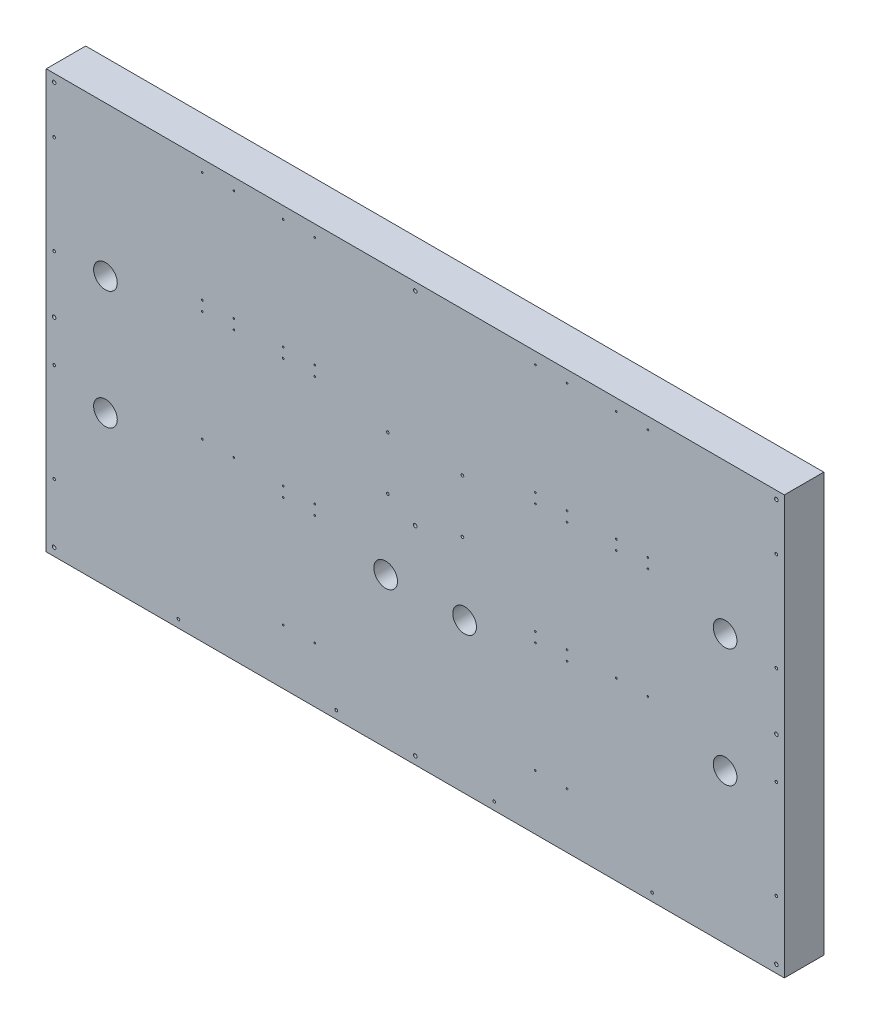
SolidWorks part; units mm, degrees
material "陶瓷"
ref_plane "前视基准面" through (0, 0, 0) normal (0, 0, 1) x (1, 0, 0)
ref_plane "上视基准面" through (0, 0, 0) normal (0, 1, 0) x (1, 0, 0)
ref_plane "右视基准面" through (0, 0, 0) normal (1, 0, 0) x (0, 0, -1)
sketch "草图1" plane through (0, 0, 0) normal (0, 0, 1) x (1, 0, 0)
  line L1 (-935, -530) -> (935, -530)
  line L2 (-935, -530) -> (-935, 530)
  line L3 (-935, 530) -> (935, 530)
  line L4 (935, -530) -> (935, 530)
  line L5 (-935, -530) -> (935, 530) construction
  line L6 (-935, 530) -> (935, -530) construction
  point P0 (0, 0)
  dimension "D1" = 1870
  dimension "D2" = 1060
extrude "凸台-拉伸1" add sketch "草图1" along normal mid plane 100
hole_wizard "M8 螺纹孔1" positions "草图2" profile "草图3" tap size "M8" standard "GB" end condition through all
sketch "草图2" plane through (0, 0, 50) normal (0, 0, 1) x (1, 0, 0)
  line L0 (-935, 530) -> (-935, -530) construction
  line L1 (-935, -530) -> (935, -530) construction
  point P0 (-69.5, 30)
  dimension "D1" = 865.5
  dimension "D2" = 560
sketch "草图3" plane through (-69.5, 30, 50) normal (1, 0, 0) x (0, -1, 0)
  line L0 (0, 0) -> (0, 100)
  line L1 (0, 100) -> (3.4, 100)
  line L2 (3.4, 100) -> (3.4, 0)
  line L5 (3.4, 0) -> (0, 0)
  line L11 (0, -6.35) -> (0, 107.95) construction
  dimension "通孔螺纹孔钻头直径" = 6.8
  dimension "通孔螺纹孔钻头深度" = 100
cosmetic thread "孔螺蚊线1" parameters "D2"=8
pattern_linear "阵列(线性)1" count 2 spacing 135 along (0, 1, 0) count 2 spacing 189 along (1, 0, 0) of "M8 螺纹孔1"
cosmetic thread "孔螺蚊线2" parameters "D2"=8
cosmetic thread "孔螺蚊线3" parameters "D2"=8
cosmetic thread "孔螺蚊线4" parameters "D2"=8
hole_wizard "打孔尺寸(%根据)内六角圆柱头螺钉的类型2" positions "草图4" profile "草图5" counterbore size "M8" standard "GB" end condition through all
sketch "草图4" plane through (0, 0, -50) normal (0, 0, -1) x (-1, 0, 0)
  line L0 (-935, -530) -> (-935, 530) construction
  line L1 (-935, 530) -> (935, 530) construction
  point P0 (-915, 510)
  dimension "D1" = 20
  dimension "D2" = 20
sketch "草图5" plane through (915, 510, -50) normal (1, 0, 0) x (0, 1, 0)
  line L0 (0, 0) -> (0, 100)
  line L1 (0, 100) -> (4.5, 100)
  line L3 (4.5, 100) -> (4.5, 50)
  line L4 (4.5, 50) -> (7.5, 50)
  line L5 (7.5, 50) -> (7.5, 0)
  line L7 (7.5, 0) -> (0, 0)
  line L11 (0, -6.35) -> (0, 107.95) construction
  dimension "通孔孔直径" = 9
  dimension "通孔孔深度" = 100
  dimension "柱形沉头孔直径" = 15
  dimension "柱形沉头孔深度" = 50
pattern_linear "阵列(线性)2" count 2 spacing 515 along (0, -1, 0) of "打孔尺寸(%根据)内六角圆柱头螺钉的类型2"
pattern_linear "阵列(线性)3" count 2 spacing 915 along (-1, 0, 0) of "打孔尺寸(%根据)内六角圆柱头螺钉的类型2", "阵列(线性)2"
hole_wizard "M5 螺纹孔1" positions "草图8" profile "草图9" tap size "M5" standard "GB" end condition through all
sketch "草图8" plane through (0, 0, -50) normal (0, 0, -1) x (-1, 0, 0)
  line L0 (-935, -530) -> (-935, 530) construction
  line L1 (-935, 530) -> (935, 530) construction
  point P0 (-589.5, 500)
  point P7 (-509.5, 500)
  dimension "D1" = 345.5
  dimension "D2" = 30
  dimension "D3" = 80
  dimension "D4" = 30
sketch "草图9" plane through (589.5, 500, -50) normal (1, 0, 0) x (0, 1, 0)
  line L0 (0, 0) -> (0, 100)
  line L1 (0, 100) -> (2.1, 100)
  line L2 (2.1, 100) -> (2.1, 0)
  line L5 (2.1, 0) -> (0, 0)
  line L11 (0, -6.35) -> (0, 107.95) construction
  dimension "通孔螺纹孔钻头直径" = 4.2
  dimension "通孔螺纹孔钻头深度" = 100
cosmetic thread "孔螺蚊线5" parameters "D2"=5
cosmetic thread "孔螺蚊线6" parameters "D2"=5
pattern_linear "阵列(线性)5" count 2 spacing 280 along (0, -1, 0) of "M5 螺纹孔1"
cosmetic thread "孔螺蚊线7" parameters "D2"=5
cosmetic thread "孔螺蚊线8" parameters "D2"=5
pattern_linear "阵列(线性)6" count 2 spacing 305 along (0, -1, 0) of "M5 螺纹孔1", "阵列(线性)5"
cosmetic thread "孔螺蚊线9" parameters "D2"=5
cosmetic thread "孔螺蚊线10" parameters "D2"=5
cosmetic thread "孔螺蚊线11" parameters "D2"=5
cosmetic thread "孔螺蚊线12" parameters "D2"=5
pattern_linear "阵列(线性)7" count 2 spacing 205 along (-1, 0, 0) of "M5 螺纹孔1", "阵列(线性)5", "阵列(线性)6"
cosmetic thread "孔螺蚊线13" parameters "D2"=5
cosmetic thread "孔螺蚊线14" parameters "D2"=5
cosmetic thread "孔螺蚊线15" parameters "D2"=5
cosmetic thread "孔螺蚊线16" parameters "D2"=5
cosmetic thread "孔螺蚊线17" parameters "D2"=5
cosmetic thread "孔螺蚊线18" parameters "D2"=5
cosmetic thread "孔螺蚊线19" parameters "D2"=5
cosmetic thread "孔螺蚊线20" parameters "D2"=5
pattern_linear "阵列(线性)8" count 2 spacing 844 along (-1, 0, 0) of "阵列(线性)7", "M5 螺纹孔1", "阵列(线性)5", "阵列(线性)6"
cosmetic thread "孔螺蚊线21" parameters "D2"=5
cosmetic thread "孔螺蚊线22" parameters "D2"=5
cosmetic thread "孔螺蚊线23" parameters "D2"=5
cosmetic thread "孔螺蚊线24" parameters "D2"=5
cosmetic thread "孔螺蚊线25" parameters "D2"=5
cosmetic thread "孔螺蚊线26" parameters "D2"=5
cosmetic thread "孔螺蚊线27" parameters "D2"=5
cosmetic thread "孔螺蚊线28" parameters "D2"=5
cosmetic thread "孔螺蚊线29" parameters "D2"=5
cosmetic thread "孔螺蚊线30" parameters "D2"=5
cosmetic thread "孔螺蚊线31" parameters "D2"=5
cosmetic thread "孔螺蚊线32" parameters "D2"=5
cosmetic thread "孔螺蚊线33" parameters "D2"=5
cosmetic thread "孔螺蚊线34" parameters "D2"=5
cosmetic thread "孔螺蚊线35" parameters "D2"=5
cosmetic thread "孔螺蚊线36" parameters "D2"=5
sketch "草图10" plane through (0, 0, -50) normal (0, 0, -1) x (-1, 0, 0)
  circle A12 centre (-304.5, -390) radius 2.1
  circle A13 centre (-384.5, -390) radius 2.1
  circle A14 centre (-304.5, -110) radius 2.1
  circle A15 centre (-384.5, -110) radius 2.1
extrude "切除-拉伸1" cut sketch "草图10" against normal through all
pattern_linear "阵列(线性)9" count 2 spacing 639 along (-1, 0, 0) of "切除-拉伸1"
sketch "草图12" plane through (0, 0, -50) normal (0, 0, -1) x (-1, 0, 0)
  line L0 (-935, -530) -> (-935, 530) construction
  line L1 (-935, 530) -> (935, 530) construction
  circle A0 centre (-785, 150) radius 30
  circle A1 centre (-785, -150) radius 30
  dimension "D1" = 60
  dimension "D4" = 60
  dimension "D6" = 300
  dimension "D2" = 150
  dimension "D3" = 380
  dimension "D5" = 150
extrude "切除-拉伸2" cut sketch "草图12" against normal through all
mirror "镜向1" about plane through (0, 0, 0) normal (1, 0, 0) of "切除-拉伸2"
mirror "镜向2" about plane through (0, 0, 0) normal (1, 0, 0) of "阵列(线性)2", "打孔尺寸(%根据)内六角圆柱头螺钉的类型2"
sketch "草图13" plane through (0, 0, -50) normal (0, 0, -1) x (-1, 0, 0)
  line L0 (935, -530) -> (-935, -530) construction
  line L1 (-935, -530) -> (-935, 530) construction
  circle A0 centre (-125, -150) radius 30
  circle A1 centre (75, -150) radius 30
  dimension "D1" = 60
  dimension "D2" = 60
  dimension "D3" = 380
  dimension "D5" = 380
  dimension "D6" = 200
  dimension "D4" = 810
extrude "切除-拉伸3" cut sketch "草图13" against normal through all
hole_wizard "M8 螺纹孔2" positions "草图14" profile "草图15" tap size "M8" standard "GB" end condition through all
sketch "草图14" plane through (0, 0, -50) normal (0, 0, -1) x (-1, 0, 0)
  line L0 (-935, 530) -> (935, 530) construction
  line L1 (-935, -530) -> (-935, 530) construction
  point P0 (-915, 390)
  dimension "D1" = 140
  dimension "D2" = 20
sketch "草图15" plane through (915, 390, -50) normal (1, 0, 0) x (0, 1, 0)
  line L0 (0, 0) -> (0, 100)
  line L1 (0, 100) -> (3.4, 100)
  line L2 (3.4, 100) -> (3.4, 0)
  line L5 (3.4, 0) -> (0, 0)
  line L11 (0, -6.35) -> (0, 107.95) construction
  dimension "通孔螺纹孔钻头直径" = 6.8
  dimension "通孔螺纹孔钻头深度" = 100
cosmetic thread "孔螺蚊线37" parameters "D2"=8
pattern_linear "阵列(线性)10" count 4 spacing 250 along (0, -1, 0) of "M8 螺纹孔2"
cosmetic thread "孔螺蚊线38" parameters "D2"=8
cosmetic thread "孔螺蚊线39" parameters "D2"=8
cosmetic thread "孔螺蚊线40" parameters "D2"=8
mirror "镜向3" about plane through (0, 0, 0) normal (1, 0, 0) of "阵列(线性)10", "M8 螺纹孔2"
cosmetic thread "孔螺蚊线41" parameters "D2"=8
cosmetic thread "孔螺蚊线42" parameters "D2"=8
cosmetic thread "孔螺蚊线43" parameters "D2"=8
cosmetic thread "孔螺蚊线44" parameters "D2"=8
hole_wizard "M8 螺纹孔3" positions "草图16" profile "草图17" tap size "M8" standard "GB" end condition through all
sketch "草图16" plane through (0, 0, -50) normal (0, 0, -1) x (-1, 0, 0)
  line L0 (-935, -530) -> (-935, 530) construction
  line L1 (935, -530) -> (-935, -530) construction
  point P0 (-600, -510)
  dimension "D1" = 335
  dimension "D2" = 20
sketch "草图17" plane through (600, -510, -50) normal (1, 0, 0) x (0, 1, 0)
  line L0 (0, 0) -> (0, 100)
  line L1 (0, 100) -> (3.4, 100)
  line L2 (3.4, 100) -> (3.4, 0)
  line L5 (3.4, 0) -> (0, 0)
  line L11 (0, -6.35) -> (0, 107.95) construction
  dimension "通孔螺纹孔钻头直径" = 6.8
  dimension "通孔螺纹孔钻头深度" = 100
cosmetic thread "孔螺蚊线45" parameters "D2"=8
pattern_linear "阵列(线性)11" count 4 spacing 400 along (-1, 0, 0) of "M8 螺纹孔3"
cosmetic thread "孔螺蚊线46" parameters "D2"=8
cosmetic thread "孔螺蚊线47" parameters "D2"=8
cosmetic thread "孔螺蚊线48" parameters "D2"=8
pattern_linear "阵列(线性)12" count 2 spacing 1020 along (0, -1, 0) of "打孔尺寸(%根据)内六角圆柱头螺钉的类型2"
pattern_linear "阵列(线性)13" count 2 spacing 915 along (-1, 0, 0) of "阵列(线性)12"
mirror "镜向4" about plane through (0, 0, 0) normal (1, 0, 0) of "阵列(线性)12"
